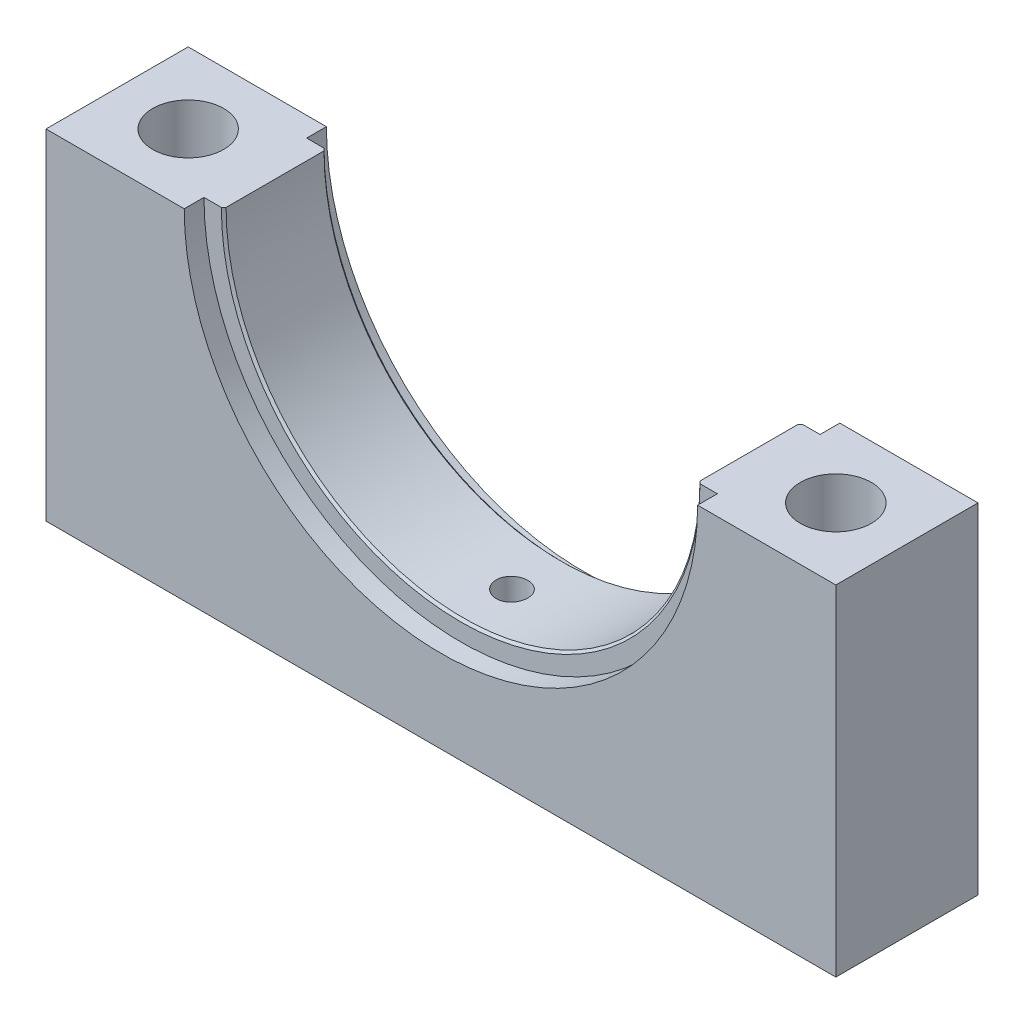
SolidWorks part; units mm, degrees
material "Q235-A"
ref_plane "Front Plane" through (0, 0, 0) normal (0, 0, 1) x (1, 0, 0)
ref_plane "Top Plane" through (0, 0, 0) normal (0, 1, 0) x (1, 0, 0)
ref_plane "Right Plane" through (0, 0, 0) normal (1, 0, 0) x (0, 0, -1)
sketch "Sketch1" plane through (0, 0, 0) normal (0, 0, 1) x (1, 0, 0)
  line L0 (-50, 0) -> (-30, 0)
  line L1 (-50, -43) -> (50, -43)
  line L2 (-50, -43) -> (-50, 0)
  line L4 (50, -43) -> (50, 0)
  line L5 (-50, -43) -> (0, 0) construction
  line L6 (22.7456, -19.5612) -> (50, -43) construction
  line L7 (30, 0) -> (50, 0)
  arc A0 (-30, 0) -> (30, 0) centre (0, 0) ccw
  point P0 (0, 0)
  dimension "D1" = 43
  dimension "D2" = 100
extrude "Boss-Extrude1" add sketch "Sketch1" along normal blind 18
sketch "Sketch2" plane through (0, 0, 18) normal (0, 0, 1) x (1, 0, 0)
  circle A0 centre (0, 0) radius 32.5
extrude "Cut-Extrude1" cut sketch "Sketch2" against normal blind 2.5
sketch "Sketch3" plane through (0, 0, 0) normal (0, 0, -1) x (-1, 0, 0)
  circle A1 centre (0, 0) radius 32.5
  circle A2 centre (0, 0) radius 32.5
  dimension "D1" = 0
extrude "Cut-Extrude2" cut sketch "Sketch3" against normal blind 2.5
chamfer "Chamfer1" distance 0.3 angle 45 2 edges at (0, -30, 2.5) (0, -30, 15.5)
sketch "Sketch4" plane through (0, 0, 0) normal (0, 1, 0) x (1, 0, 0)
  line L0 (-41, -9) -> (41, -9)
  line L1 (-50, -18) -> (-50, 0) construction
  line L2 (50, 0) -> (32.5, 0) construction
  dimension "D1" = 82
  dimension "D2" = 9
  dimension "D3" = 9
hole_wizard "Hole1" positions "Sketch5" profile "Sketch6" legacy end condition through all
sketch "Sketch5" plane through (0, 0, 0) normal (0, 1, 0) x (1, 0, 0)
  point P0 (-41, -9)
  point P3 (41, -9)
sketch "Sketch6" plane through (-41, 0, 9) normal (1, 0, 0) x (0, 0, 1)
  line L0 (0, 0) -> (0, 43)
  line L1 (0, 43) -> (4.5, 43)
  line L2 (4.5, 43) -> (4.5, 0)
  line L3 (4.5, 0) -> (0, 0)
  line L4 (0, 110) -> (0, -10) construction
  dimension "直径" = 9
  dimension "深度" = 43
sketch "Sketch8" plane through (0, 0, 0) normal (0, 1, 0) x (1, 0, 0)
  line L0 (0, -18) -> (0, 0)
  line L1 (-32.5, -18) -> (32.5, -18) construction
  line L2 (32.5, 0) -> (-32.5, 0) construction
hole_wizard "Hole2" positions "Sketch9" profile "Sketch10" legacy
sketch "Sketch9" plane through (0, 0, 0) normal (0, 1, 0) x (1, 0, 0)
  line L0 (0, -18) -> (0, 0) construction
  point P0 (0, -9)
sketch "Sketch10" plane through (0, 0, 9) normal (1, 0, 0) x (0, 0, 1)
  line L0 (0, 0) -> (0, 34)
  line L1 (0, 34) -> (2, 34)
  line L2 (2, 34) -> (2, 0)
  line L3 (2, 0) -> (0, 0)
  line L4 (0, 110) -> (0, -10) construction
  dimension "直径" = 4
  dimension "深度" = 34
